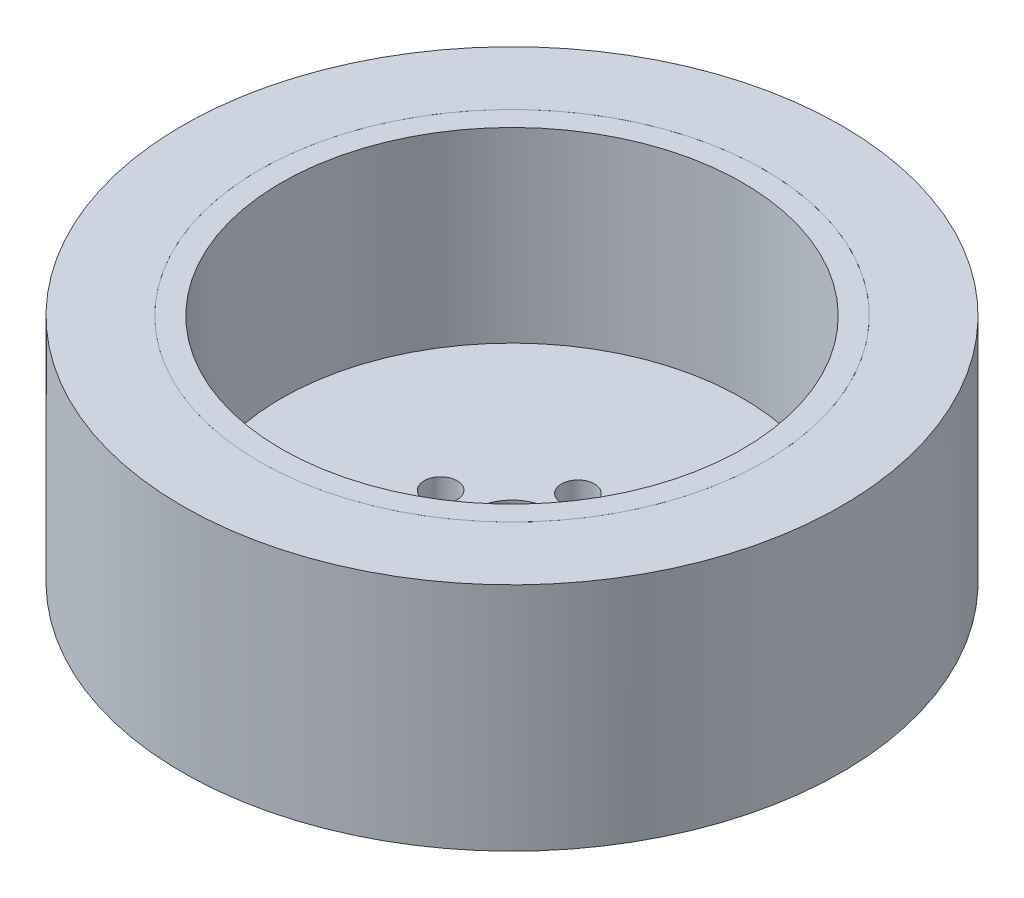
SolidWorks part; units mm, degrees
other "包胶"
other "轮毂"
ref_plane "前视基准面" through (0, 0, 0) normal (0, 0, 1) x (1, 0, 0)
ref_plane "上视基准面" through (0, 0, 0) normal (0, 1, 0) x (1, 0, 0)
ref_plane "右视基准面" through (0, 0, 0) normal (1, 0, 0) x (0, 0, -1)
sketch "轮毂形体定义" plane through (0, 0, 0) normal (0, 1, 0) x (1, 0, 0)
  line L0 (-6.5, 0) -> (6.5, 0) construction
  line L1 (0, 6) -> (0, -6) construction
  circle A0 centre (0, 0) radius 23
  circle A1 centre (0, 0) radius 3.5
  circle A2 centre (0, 0) radius 21 construction
  circle A3 centre (0, 6) radius 1.5
  circle A4 centre (0, -6) radius 1.5
  circle A5 centre (-6.5, 0) radius 1.5
  circle A6 centre (6.5, 0) radius 1.5
  dimension "D1" = 46
  dimension "D2" = 42
  dimension "D3" = 12
  dimension "D5" = 3
  dimension "D6" = 7
  dimension "D4" = 13
sketch "草图1" plane through (0, 0, 0) normal (0, 1, 0) x (1, 0, 0)
  circle A9 centre (6.5, 0) radius 1.5
  circle A10 centre (6.5, 0) radius 1.5
  circle A11 centre (-6.5, 0) radius 1.5
  circle A12 centre (-6.5, 0) radius 1.5
  circle A13 centre (0, -6) radius 1.5
  circle A14 centre (0, -6) radius 1.5
  circle A15 centre (0, 6) radius 1.5
  circle A16 centre (0, 6) radius 1.5
  circle A17 centre (0, 0) radius 3.5
  circle A18 centre (0, 0) radius 3.5
  circle A19 centre (0, 0) radius 23
  circle A20 centre (0, 0) radius 23
  dimension "D1" = 0
  dimension "D3" = 0
  dimension "D4" = 0
  dimension "D5" = 0
  dimension "D6" = 0
  dimension "D2" = 0
extrude "凸台-拉伸1" add sketch "草图1" along normal blind 4
sketch "草图2" plane through (0, 4, 0) normal (0, 1, 0) x (1, 0, 0)
  circle A0 centre (0, 0) radius 21 construction
  circle A1 centre (0, 0) radius 21
  circle A15 centre (0, 0) radius 23
  circle A16 centre (0, 0) radius 23
  dimension "D6" = 0
extrude "凸台-拉伸2" add sketch "草图2" along normal blind 17
sketch "草图3" plane through (0, 0, 0) normal (0, -1, 0) x (1, 0, 0)
  circle A2 centre (0, 0) radius 30
  circle A14 centre (0, 0) radius 23
  circle A15 centre (0, 0) radius 23
  point P0 (0, 0)
  dimension "D1" = 60
  dimension "D7" = 0
extrude "凸台-拉伸3" add sketch "草图3" against normal up to surface (21 mm away) separate body up to face at (0, 21, 23)
